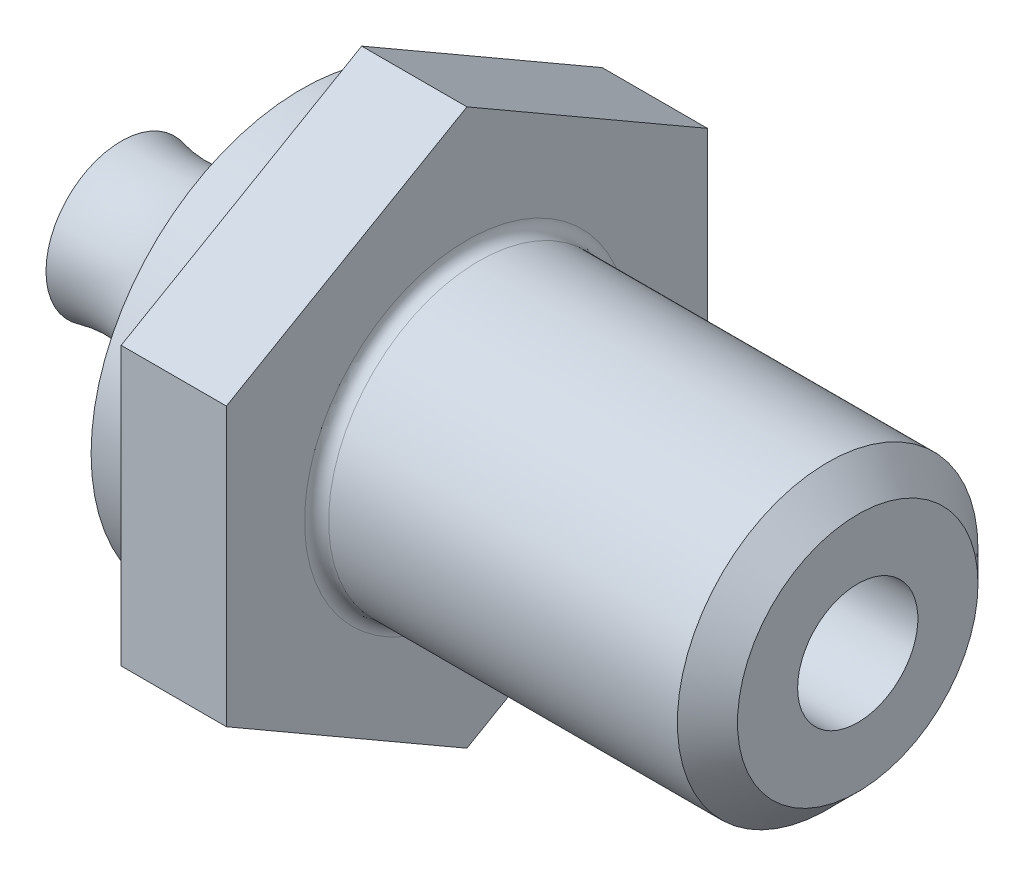
from build123d import *

# Parameters (mm, degrees)
BASE_EXTRUDE_DEPTH      = 6.4
FILLET_2_R              = 0.4
CUT_EXTRUDE1_DEPTH      = 23.928003257
CUT_EXTRUDE1_DEPTH_BACK = 23.928003257
SKETCH8_W               = 2.9
SKETCH8_H               = 16


with BuildPart() as part:
    # Sketch1 → Base-Extrude (new body)
    with BuildSketch(Plane(origin=(0, 0, 0), x_dir=(0, 0, -1), z_dir=(1, 0, 0))):
        Polygon((8, 4.618802154), (8, -4.618802154), (0, -9.237604307), (-8, -4.618802154), (-8, 4.618802154), (0, 9.237604307), align=None)
    extrude(amount=BASE_EXTRUDE_DEPTH)

    # Sketch2 → Boss-Revolve1 (revolve)
    with BuildSketch(Plane.XY, mode=Mode.PRIVATE) as boss_revolve1_sk:
        Polygon((0, 0), (32.4, 0), (32.4, 4.134), (32.4, 5), (27.8072, 5), (0, 5), align=None)
    revolve(boss_revolve1_sk.sketch.rotate(Axis((0, 0, 0), (1, 0, 0)), 90), axis=Axis((0, 0, 0), (1, 0, 0)))

    # Sketch3 → Cut-Revolve1 (revolve, cut)
    with BuildSketch(Plane.XY):
        Polygon((0, 8), (3.601282526, 14.237604307), (3.601282526, 19.237604307), (-10, 19.237604307), (-10, 8), align=None)
    revolve(axis=Axis((0, 0, 0), (1, 0, 0)), mode=Mode.SUBTRACT)

    # Fillet 2
    fillet_2_edges = [part.edges().sort_by_distance(p)[0] for p in [
        (6.4, 0, -5),
    ]]
    fillet(fillet_2_edges, radius=FILLET_2_R)

    # Sketch7 → Cut-Revolve5 (revolve, cut)
    with BuildSketch(Plane(origin=(0, 0, 0), x_dir=(1, 0, 0), z_dir=(0, 1, 0))):
        Polygon((32.4, 5), (18.4, 5), (19.4, 4), (19.4, 0), (32.4, 0), align=None)
    revolve(axis=Axis((34.209458749, 0, 0), (-1, 0, 0)), mode=Mode.SUBTRACT)

    # Sketch8 → Cut-Extrude1 (cut, two sides: drawn at the far end of the back side and taken through both)
    with BuildSketch(Plane(origin=(0, 0, 0), x_dir=(1, 0, 0), z_dir=(0, 1, 0)).offset(-CUT_EXTRUDE1_DEPTH_BACK)):
        with Locations((1.45, 0)):
            Rectangle(SKETCH8_W, SKETCH8_H)
    extrude(amount=CUT_EXTRUDE1_DEPTH + CUT_EXTRUDE1_DEPTH_BACK, mode=Mode.SUBTRACT)

    # Sketch9 → Revolve1 (revolve)
    with BuildSketch(Plane(origin=(0, 0, 0), x_dir=(1, 0, 0), z_dir=(0, 1, 0))):
        with BuildLine():
            Line((-5.1, 0), (-5.1, 2.5))
            ThreePointArc((-5.1, 2.5), (-1.393005283, 3.038009057), (0.9, 6))
            Line((0.9, 6), (0.9, 7))
            Line((0.9, 7), (2.9, 7))
            Line((2.9, 7), (2.9, 0))
            Line((2.9, 0), (-5.1, 0))
        make_face()
    revolve(axis=Axis((-7.317514451, 0, 0), (1, 0, 0)))

    # Sketch10 → Cut-Revolve6 (revolve, cut)
    with BuildSketch(Plane(origin=(0, 0, 0), x_dir=(1, 0, 0), z_dir=(0, 1, 0)), mode=Mode.PRIVATE) as cut_revolve6_sk:
        with BuildLine():
            Line((19.4, 0), (19.4, 2))
            Line((19.4, 2), (-0.22471637, 2))
            Line((-0.22471637, 2), (-0.22471637, 1.5))
            Line((-0.22471637, 1.5), (-4.1, 1.5))
            ThreePointArc((-4.1, 1.5), (-4.635233135, 1.401258538), (-5.1, 1.118033989))
            Line((-5.1, 1.118033989), (-5.1, 0))
            Line((-5.1, 0), (19.4, 0))
        make_face()
    revolve(cut_revolve6_sk.sketch.rotate(Axis((-5.799172577, 0, 0), (1, 0, 0)), 180), axis=Axis((-5.799172577, 0, 0), (1, 0, 0)), mode=Mode.SUBTRACT)


solid = part.part
